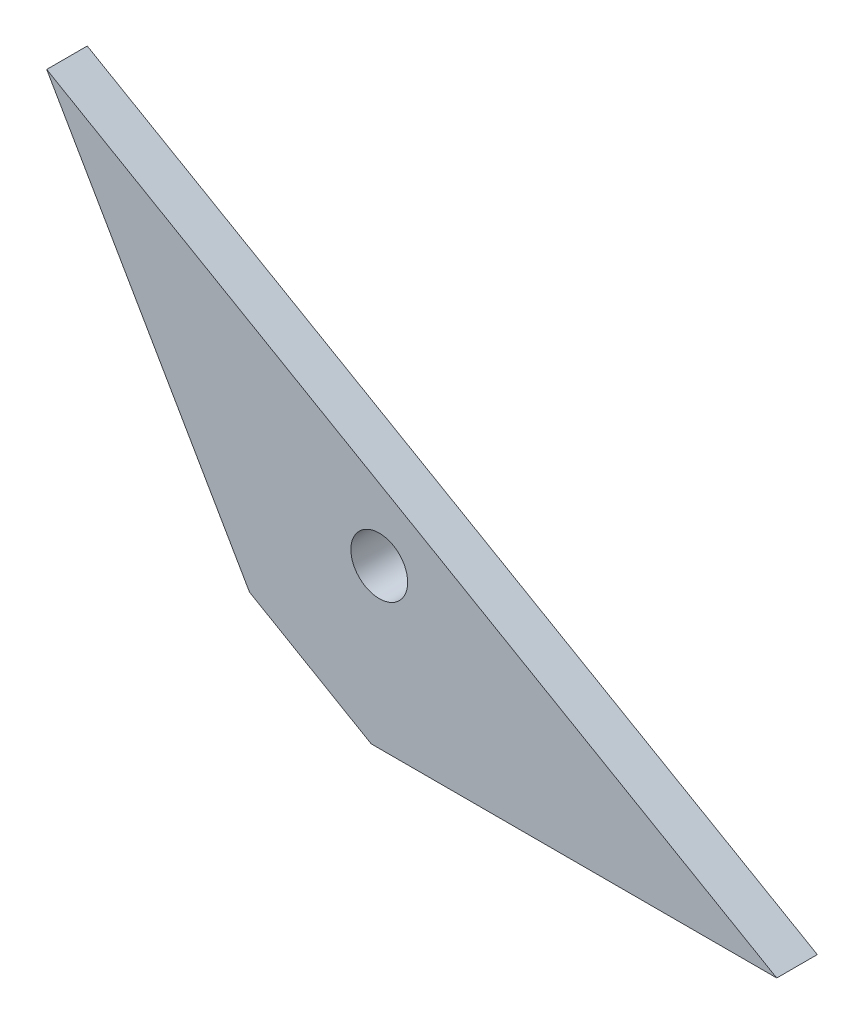
from build123d import *

# Parameters (mm, degrees)
SKETCH1_R           = 7
BOSS_EXTRUDE1_DEPTH = 10


with BuildPart() as part:
    # Sketch1 → Boss-Extrude1 (new body)
    with BuildSketch(Plane.XY):
        Polygon((-80, 104), (-30, 17.397459622), (0, 0), (100, 0), align=None)
        with Locations((2, 39)):
            Circle(SKETCH1_R, mode=Mode.SUBTRACT)
    extrude(amount=BOSS_EXTRUDE1_DEPTH)


solid = part.part
